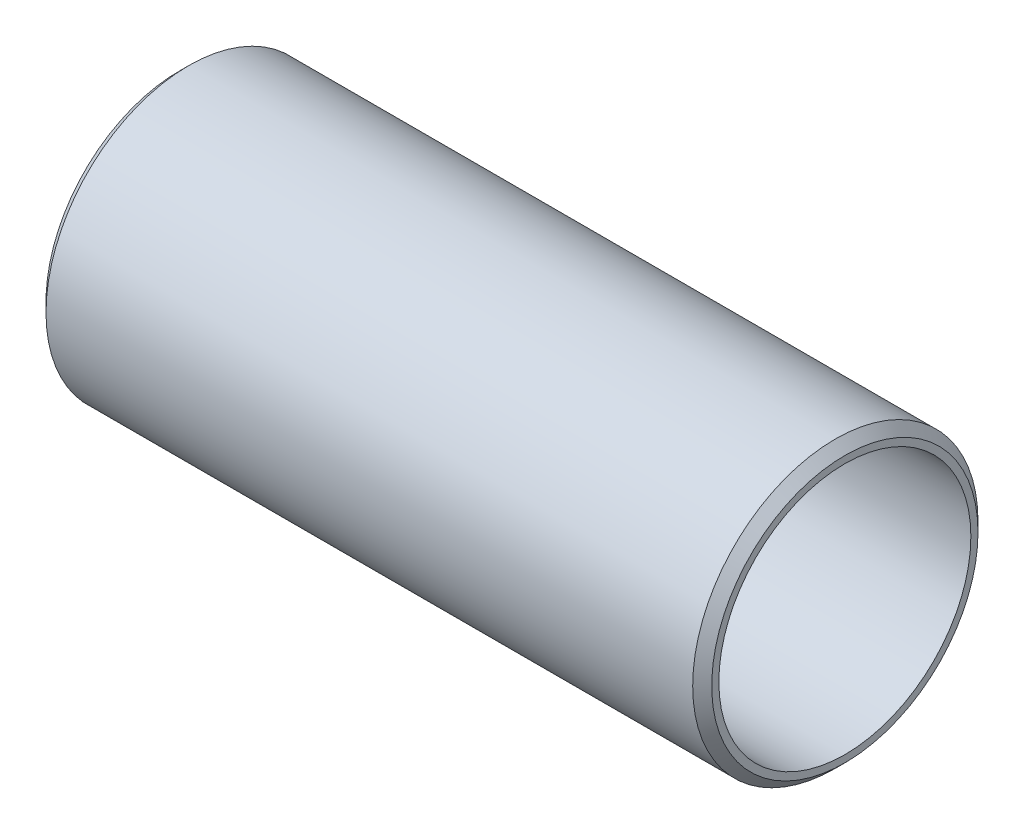
from build123d import *

# Parameters (mm, degrees)
SKETCH_1_R      = 30
SKETCH_1_R_2    = 26.5
EXTRUDE_1_DEPTH = 140
CHAMFER_1_SIZE  = 2


with BuildPart() as part:
    # 草图1 → 拉伸-薄壁1 (new body)
    with BuildSketch(Plane(origin=(0, 0, 0), x_dir=(0, 0, -1), z_dir=(1, 0, 0))):
        Circle(SKETCH_1_R)
        Circle(SKETCH_1_R_2, mode=Mode.SUBTRACT)
    extrude(amount=EXTRUDE_1_DEPTH)

    # 倒角1
    chamfer_1_edges = [part.edges().sort_by_distance(p)[0] for p in [
        (0, 0, 30),
        (140, 0, 30),
    ]]
    chamfer(chamfer_1_edges, length=CHAMFER_1_SIZE)


solid = part.part
